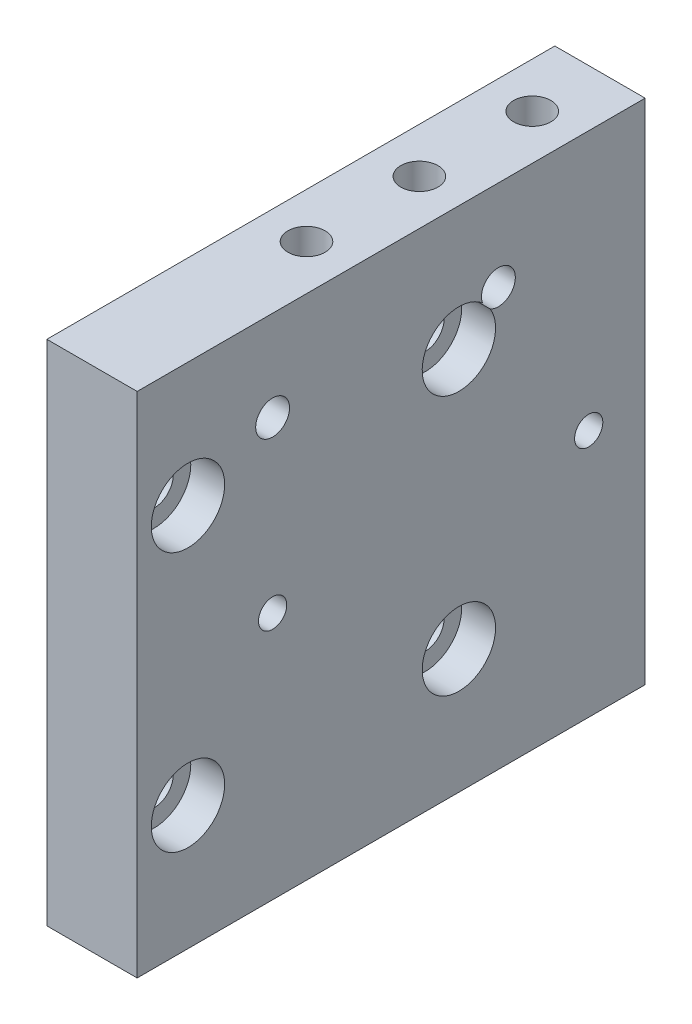
SolidWorks part; units mm, degrees
material "6061 Alloy"
ref_plane "Front Plane" through (0, 0, 0) normal (0, 0, 1) x (1, 0, 0)
ref_plane "Top Plane" through (0, 0, 0) normal (0, 1, 0) x (1, 0, 0)
ref_plane "Right Plane" through (0, 0, 0) normal (1, 0, 0) x (0, 0, -1)
sketch "Sketch 1" plane through (0, 0, 0) normal (1, 0, 0) x (0, 0, -1)
  line L1 (-22.5, -22.5) -> (22.5, -22.5)
  line L2 (-22.5, -22.5) -> (-22.5, 22.5)
  line L3 (-22.5, 22.5) -> (22.5, 22.5)
  line L4 (22.5, -22.5) -> (22.5, 22.5)
  line L5 (-22.5, -22.5) -> (22.5, 22.5) construction
  line L6 (-22.5, 22.5) -> (22.5, -22.5) construction
  point P0 (0, 0)
  dimension "D1" = 45
  dimension "D2" = 45
extrude "Boss-Extrude 1" add sketch "Sketch 1" along normal blind 8
hole_wizard "M3 Hex Socket Cap Screw Counterbore 1" positions "Sketch 3" profile "Sketch 2" counterbore size "M3" standard "ISO" end condition through all
sketch "Sketch 3" plane through (8, 0, 0) normal (1, 0, 0) x (0, 0, -1)
  line L0 (22.5, 22.5) -> (-22.5, 22.5) construction
  line L1 (-22.5, 22.5) -> (-22.5, -22.5) construction
  point P0 (-18, 11.5)
  dimension "D1" = 11
  dimension "D2" = 4.5
sketch "Sketch 2" plane through (8, 11.5, 18) normal (0, 1, 0) x (0, 0, -1)
  line L0 (0, 0) -> (0, 8)
  line L1 (0, 8) -> (1.7, 8)
  line L3 (1.7, 8) -> (1.7, 3)
  line L4 (1.7, 3) -> (3.25, 3)
  line L5 (3.25, 3) -> (3.25, 0)
  line L7 (3.25, 0) -> (0, 0)
  line L11 (0, -6.35) -> (0, 107.95) construction
  dimension "貫穿孔直徑" = 3.4
  dimension "貫穿孔深度" = 8
  dimension "柱孔直徑" = 6.5
  dimension "柱孔深度" = 3
pattern_linear "Linear Pattern 1" count 2 spacing 23 along (0, -1, 0) of "M3 Hex Socket Cap Screw Counterbore 1"
pattern_linear "Linear Pattern 2" count 2 spacing 24 along (0, 0, -1) of "Linear Pattern 1", "M3 Hex Socket Cap Screw Counterbore 1"
hole_wizard "M4 Tapped Hole 1" positions "Sketch 7" profile "Sketch 6" tap size "M4" standard "GB"
sketch "Sketch 7" plane through (0, 22.5, 0) normal (0, 1, 0) x (-1, 0, 0)
  line L1 (-8, -22.5) -> (-8, 22.5) construction
  line L2 (-8, -22.5) -> (0, -22.5) construction
  point P0 (-4, -16.5)
  dimension "D1" = 6
  dimension "D2" = 4
sketch "Sketch 6" plane through (4, 22.5, -16.5) normal (1, 0, 0) x (0, 0, 1)
  line L0 (0, 0) -> (0, 11.0914)
  line L1 (0, 11.0914) -> (1.65, 10.1)
  line L2 (1.65, 10.1) -> (1.65, 0)
  line L5 (1.65, 0) -> (0, 0)
  line L10 (0, 11.0914) -> (-1.65, 10.1) construction
  line L11 (0, -6.35) -> (0, 107.95) construction
  dimension "螺孔鑽直徑" = 3.3
  dimension "螺孔鑽深度" = 10.1
  dimension "導頭角度" = 118
cosmetic thread "Cosmetic Thread 2" parameters "D1"=8, "D2"=4
pattern_linear "Linear Pattern 5" count 3 spacing 10 along (0, 0, 1) of "M4 Tapped Hole 1"
hole_wizard "M3 Tapped Hole 1" positions "Sketch 9" profile "Sketch 8" tap size "M3" standard "GB" end condition through all
sketch "Sketch 9" plane through (8, 0, 0) normal (1, 0, 0) x (0, 0, -1)
  line L0 (22.5, 22.5) -> (-22.5, 22.5) construction
  line L2 (22.5, -22.5) -> (22.5, 22.5) construction
  point P0 (17.5, -0.5)
  dimension "D1" = 23
  dimension "D2" = 5
sketch "Sketch 8" plane through (8, -0.5, -17.5) normal (0, 1, 0) x (0, 0, -1)
  line L0 (0, 0) -> (0, 8)
  line L1 (0, 8) -> (1.25, 8)
  line L2 (1.25, 8) -> (1.25, 0)
  line L5 (1.25, 0) -> (0, 0)
  line L11 (0, -6.35) -> (0, 107.95) construction
  dimension "貫穿螺孔鑽直徑" = 2.5
  dimension "貫穿螺孔鑽深度" = 8
cosmetic thread "Cosmetic Thread 3" parameters "D2"=3
pattern_linear "Linear Pattern 6" count 2 spacing 28 along (0, 0, 1) of "M3 Tapped Hole 1"
hole_wizard "Ø3.0 (3) Hole 1" positions "Sketch 11" profile "Sketch 10" hole size "Ø3.0" standard "GB" end condition through all
sketch "Sketch 11" plane through (8, 0, 0) normal (1, 0, 0) x (0, 0, -1)
  circle A2 centre (-10.5, -0.5) radius 1.25 construction
  point P0 (-10.5, 14.5)
  dimension "D2" = 15
  dimension "D1" = 0
sketch "Sketch 10" plane through (8, 14.5, 10.5) normal (0, 1, 0) x (0, 0, -1)
  line L0 (0, 0) -> (0, 8)
  line L1 (0, 8) -> (1.5, 8)
  line L2 (1.5, 8) -> (1.5, 0)
  line L5 (1.5, 0) -> (0, 0)
  line L11 (0, -6.35) -> (0, 107.95) construction
  dimension "貫穿孔直徑" = 3
  dimension "貫穿孔深度" = 8
pattern_linear "Linear Pattern 8" count 2 spacing 20 along (0, 0, -1) of "Ø3.0 (3) Hole 1"
